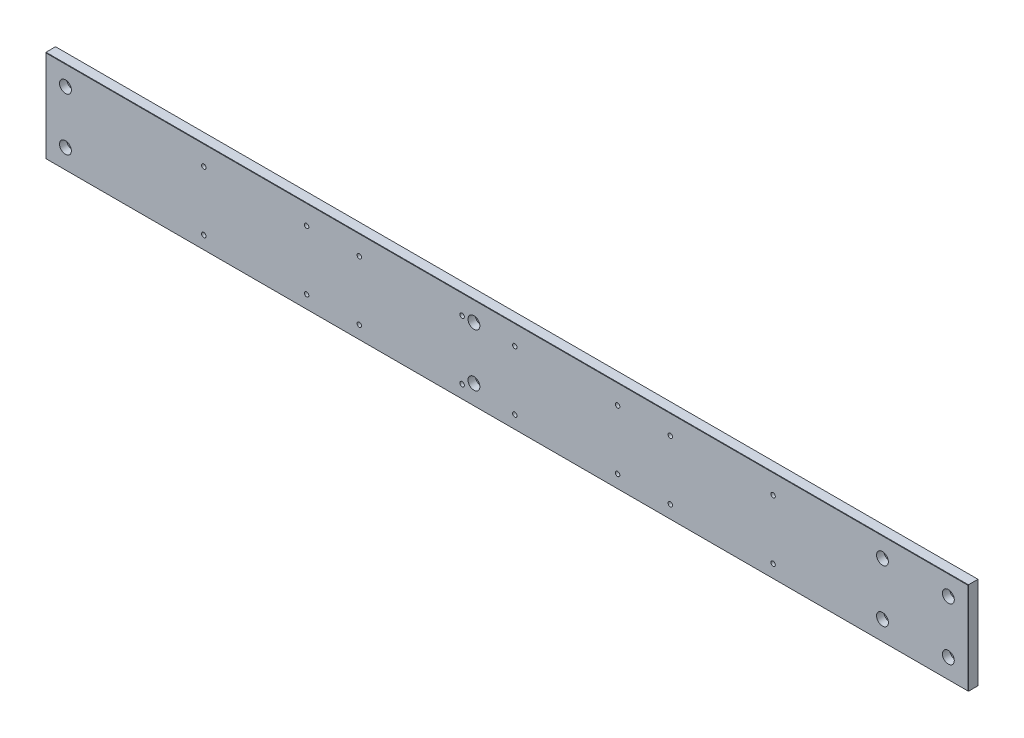
from build123d import *

# Parameters (mm, degrees)
SKETCH_1_W                  = 1400
SKETCH_1_H                  = 140
EXTRUDE_1_DEPTH             = 7.5
HOLE_WIZARD_1_D             = 11
HOLE_WIZARD_1_CBORE_D       = 18
HOLE_WIZARD_1_CBORE_DEPTH   = 11
PATTERN_LINEAR_1_COUNT      = 3
PATTERN_LINEAR_1_PITCH      = 620
PATTERN_LINEAR_1_COUNT_DIR2 = 2
PATTERN_LINEAR_1_PITCH_DIR2 = 80
HOLE_WIZARD_2_D             = 11
HOLE_WIZARD_2_CBORE_D       = 18
HOLE_WIZARD_2_CBORE_DEPTH   = 11
CHAMFER_1_SIZE              = 0.5
HOLE_WIZARD_M8_1_D          = 6.8


with BuildPart() as part:
    # 草图1 → 凸台-拉伸1 (new, symmetric)
    with BuildSketch(Plane.XY):
        Rectangle(SKETCH_1_W, SKETCH_1_H)
    extrude(amount=EXTRUDE_1_DEPTH, both=True)

    # 打孔尺寸(%根据)内六角圆柱头螺钉的类型1 (through all)
    with Locations(Plane(origin=(-670, 40, 7.5), x_dir=(1, 0, 0), z_dir=(0, 0, 1))):
        with Locations((0, 0)):
            hole_wizard_1 = CounterBoreHole(HOLE_WIZARD_1_D / 2, HOLE_WIZARD_1_CBORE_D / 2, HOLE_WIZARD_1_CBORE_DEPTH)

    # 阵列(线性)1: Hole Wizard 1 3 × 2
    with Locations(*[(i * PATTERN_LINEAR_1_PITCH, -j * PATTERN_LINEAR_1_PITCH_DIR2, 0) for i in range(PATTERN_LINEAR_1_COUNT) for j in range(PATTERN_LINEAR_1_COUNT_DIR2) if (i, j) != (0, 0)]):
        add(hole_wizard_1, mode=Mode.SUBTRACT)

    # 打孔尺寸(%根据)内六角圆柱头螺钉的类型2 (through all)
    with Locations(Plane(origin=(670, 40, 7.5), x_dir=(1, 0, 0), z_dir=(0, 0, 1))):
        with Locations((0, 0), (0, -80)):
            CounterBoreHole(HOLE_WIZARD_2_D / 2, HOLE_WIZARD_2_CBORE_D / 2, HOLE_WIZARD_2_CBORE_DEPTH)

    # 倒角1
    chamfer_1_edges = [part.edges().sort_by_distance(p)[0] for p in [
        (-700, 0, 7.5),
        (0, -70, 7.5),
        (700, 0, 7.5),
        (0, 70, 7.5),
    ]]
    chamfer(chamfer_1_edges, length=CHAMFER_1_SIZE)

    # M8 螺纹孔1 (through all)
    with Locations(Plane.XY.offset(7.5)):
        with Locations((-460, 40), (-460, -50), (-304, -50), (-304, 40), (-224, 40), (-224, -50), (-68, -50), (-68, 40), (12, 40), (12, -50), (168, -50), (168, 40), (248, 40), (248, -50), (404, -50), (404, 40)):
            Hole(HOLE_WIZARD_M8_1_D / 2)


solid = part.part
